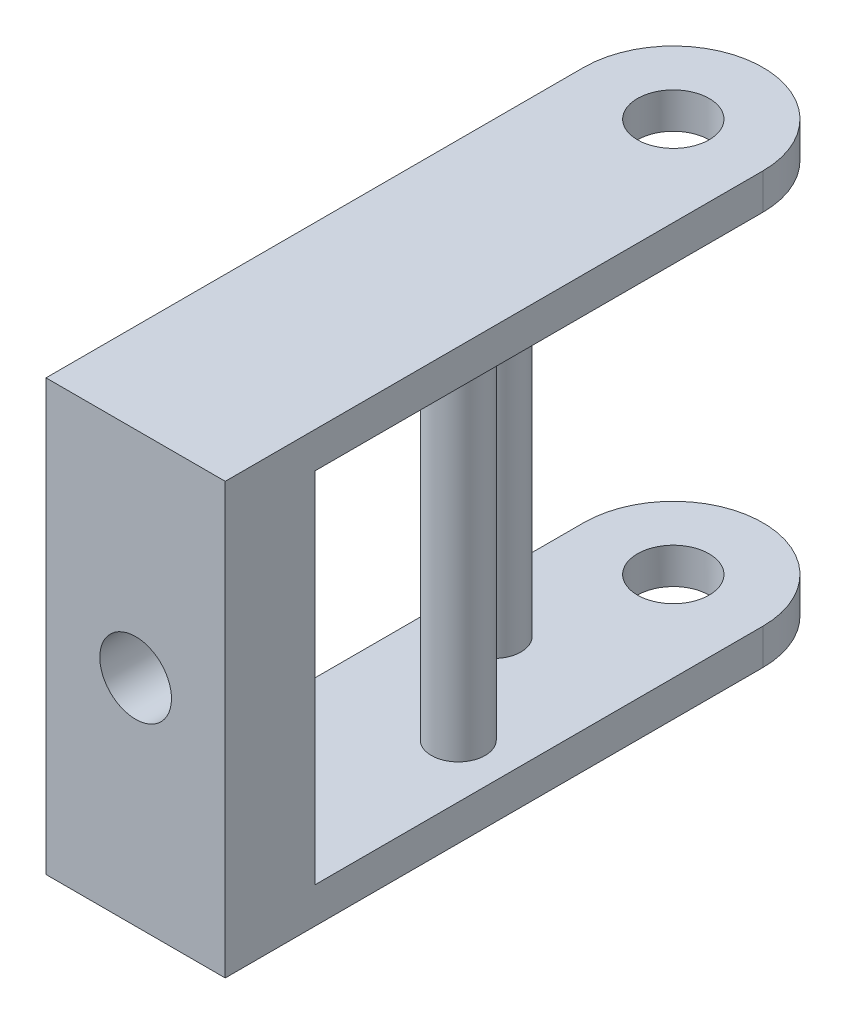
SolidWorks part; units mm, degrees
ref_plane "Front Plane" through (0, 0, 0) normal (0, 0, 1) x (1, 0, 0)
ref_plane "Top Plane" through (0, 0, 0) normal (0, 1, 0) x (1, 0, 0)
ref_plane "Right Plane" through (0, 0, 0) normal (1, 0, 0) x (0, 0, -1)
other "Configuration Table"
sketch "Sketch1" plane through (0, 0, 0) normal (0, 1, 0) x (1, 0, 0)
  line L0 (-5, 0) -> (-5, -30)
  line L1 (0, -3.85) -> (0, 3.85) construction
  line L2 (5, 0) -> (5, -30)
  line L3 (-5, -30) -> (5, -30)
  arc A0 (5, 0) -> (-5, 0) centre (0, 0) ccw
  dimension "D1" = 10
  dimension "D2" = 30
extrude "Boss-Extrude1" add sketch "Sketch1" along normal blind 24
sketch "Sketch4" plane through (0, 24, 0) normal (0, 1, 0) x (1, 0, 0)
  circle A0 centre (0, 0) radius 2
  dimension "D1" = 4
extrude "Cut-Extrude2" cut sketch "Sketch4" against normal through all both and the other way through all
sketch "Sketch6" plane through (0, 0, 0) normal (1, 0, 0) x (0, 0, -1)
  line L0 (-25, 22) -> (-25, 2)
  line L1 (-25, 2) -> (7.5888, 2)
  line L2 (7.5888, 2) -> (7.5888, 22)
  line L3 (7.5888, 22) -> (-25, 22)
  line L4 (-30, 24) -> (-30, 0) construction
  line L5 (-30, 24) -> (0, 24) construction
  line L6 (-30, 0) -> (0, 0) construction
  dimension "D1" = 5
  dimension "D2" = 2
  dimension "D3" = 2
extrude "Cut-Extrude3" cut sketch "Sketch6" against normal through all both and the other way through all
sketch "Sketch7" plane through (0, 0, 25) normal (0, 0, -1) x (-1, 0, 0)
  line L0 (0, 24) -> (0, 0) construction
  line L1 (5, 24) -> (-5, 24) construction
  circle A0 centre (0, 12) radius 2
  dimension "D1" = 4
extrude "Cut-Extrude4" cut sketch "Sketch7" against normal through all
sketch "Sketch8" plane through (0, 24, 0) normal (0, 1, 0) x (1, 0, 0)
  line L0 (-5, 0) -> (-5, -30) construction
  line L2 (5, -30) -> (5, 0) construction
  circle A0 centre (-2, -8) radius 1.5
  circle A1 centre (2, -14) radius 1.5
  dimension "D2" = 3
  dimension "D3" = 3
  dimension "D4" = 14
  dimension "D5" = 3
  dimension "D6" = 3
  dimension "D1" = 8
extrude "Boss-Extrude3" add sketch "Sketch8" against normal up to surface (22 mm away) up to face at (0, 2, -2)
